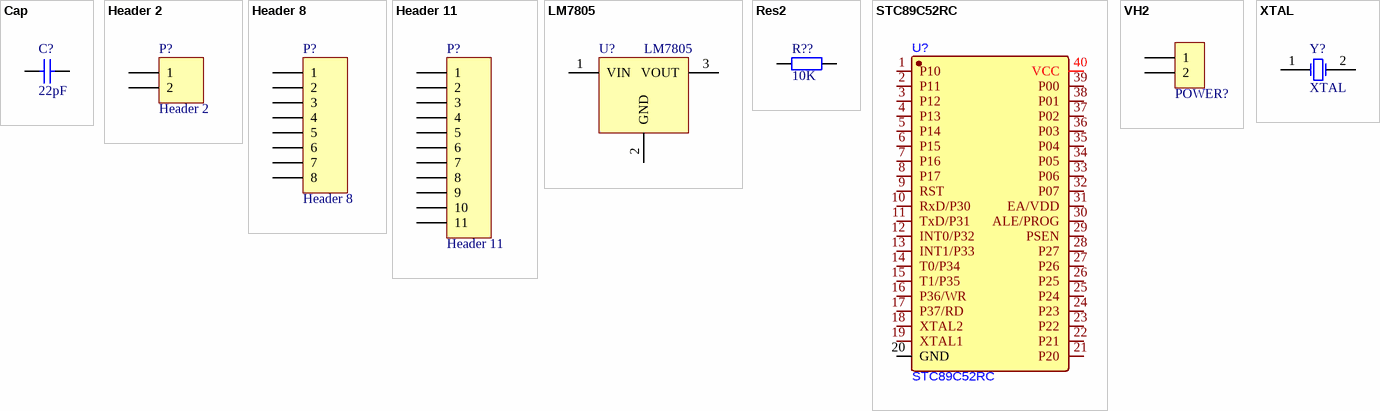
[diagram p0: symbols Cap to XTAL]
# Altium schematic symbol library MISC80518-3.SchLib: 9 symbols
Pins are listed as number, name and electrical type; pins without a type are passive.


## Cap
designator C?, comment 22pF
Capacitor; Value: 100pF
footprint RAD-0.3 (Radial Cap, Thru-Hole; 2 Leads; 0.3 in Pin Spacing)
simulation model CAP (Capacitor)
signal-integrity model Cap
pins: 1, 2

## Header 2
designator P?
Header, 2-Pin
footprint HDR1X2 (Connector; Header; 2 Position)
signal-integrity model Connector
pins: 1, 2

## Header 8
designator P?
Header, 8-Pin
footprint HDR1X8 (Connector; Header; 8 Position)
signal-integrity model Connector
pins: 1, 2, 3, 4, 5, 6, 7, 8

## Header 11
designator P?
Header, 11-Pin
footprint HDR1X11 (Connector; Header; 11 Position)
signal-integrity model Connector
pins: 1, 2, 3, 4, 5, 6, 7, 8, 9, 10, 11

## LM7805
designator U?
footprint TO220A (220, 3-pin transistor)
footprint TO252 (252 transistor)
pins: 1 VIN, 2 GND, 3 VOUT

## Res2
designator R??, comment 10K
Resistor; Value: 1K
footprint AXIAL-0.4 (Axial Device, Thru-Hole; 2 Leads; 0.4 in Pin Spacing)
simulation model RESISTOR (Resistor)
signal-integrity model Res
pins: 1, 2

## STC89C52RC
designator U?
footprint STC89C52RC
pins: 1 P10, 2 P11, 3 P12, 4 P13, 5 P14, 6 P15, 7 P16, 8 P17, 9 RST, 10 RxD/P30, 11 TxD/P31, 12 INT0/P32, 13 INT1/P33, 14 T0/P34, 15 T1/P35, 16 P36/WR, 17 P37/RD, 18 XTAL2, 19 XTAL1, 20 GND, 21 P20, 22 P21, 23 P22, 24 P23, 25 P24, 26 P25, 27 P26, 28 P27, 29 PSEN, 30 ALE/PROG, 31 EA/VDD, 32 P07, 33 P06, 34 P05, 35 P04, 36 P03, 37 P02, 38 P01, 39 P00, 40 VCC

## VH2
designator POWER?, comment Terminal block  (value not drawn)
footprint VH3.96-2A
footprint VH3.96-2AW
footprint VH3.96-2AWD
pins: 1, 2

## XTAL
designator Y?
Crystal Oscillator
footprint R38 (Crystal, Thru-Hole; 2 Leads; Body 3.1 x 8.2 mm (Dia.xH))
simulation model XTAL (Spice Subcircuit)
pins: 1 OSC1, 2 OSC2